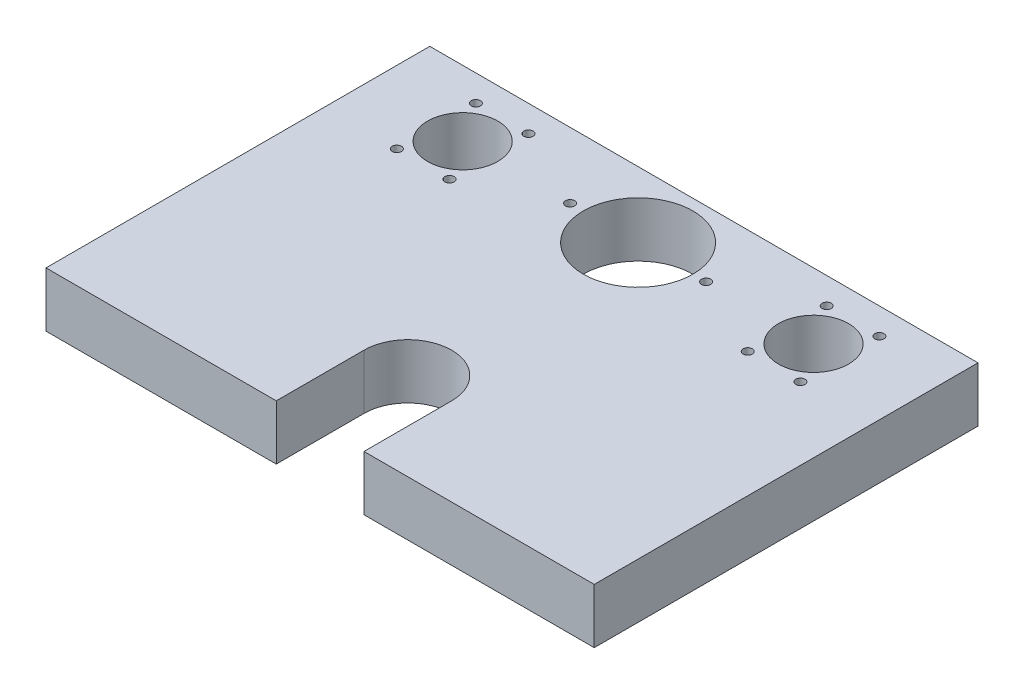
SolidWorks part; units mm, degrees
ref_plane "Front Plane" through (0, 0, 0) normal (0, 0, 1) x (1, 0, 0)
ref_plane "Top Plane" through (0, 0, 0) normal (0, 1, 0) x (1, 0, 0)
ref_plane "Right Plane" through (0, 0, 0) normal (1, 0, 0) x (0, 0, -1)
sketch "Sketch1" plane through (0, 0, 0) normal (0, 1, 0) x (1, 0, 0)
  line L1 (-125, 87.5) -> (125, 87.5)
  line L2 (-125, 87.5) -> (-125, -87.5)
  line L3 (-125, -87.5) -> (125, -87.5)
  line L4 (125, 87.5) -> (125, -87.5)
  line L5 (-125, 87.5) -> (125, -87.5) construction
  line L6 (-125, -87.5) -> (125, 87.5) construction
  point P0 (0, 0)
  dimension "D1" = 250
  dimension "D2" = 175
extrude "Boss-Extrude1" add sketch "Sketch1" along normal blind 25
sketch "Sketch2" plane through (0, 25, 0) normal (0, 1, 0) x (1, 0, 0)
  line L0 (-20, -47.5) -> (-20, -87.5)
  line L1 (-125, -87.5) -> (125, -87.5) construction
  line L2 (-20, -87.5) -> (20, -87.5)
  line L3 (20, -87.5) -> (20, -47.5)
  arc A0 (20, -47.5) -> (-20, -47.5) centre (0, -47.5) ccw
  dimension "D1" = 40
  dimension "D2" = 40
extrude "Cut-Extrude1" cut sketch "Sketch2" against normal through all
sketch "Sketch3" plane through (0, 25, 0) normal (0, 1, 0) x (1, 0, 0)
  line L0 (0, 0) -> (0, 48.5331) construction
  line L1 (125, 87.5) -> (-125, 87.5) construction
  circle A0 centre (-80, 57.5) radius 16
  circle A1 centre (80, 57.5) radius 16
  dimension "D1" = 32
  dimension "D2" = 30
  dimension "D3" = 80
extrude "Cut-Extrude2" cut sketch "Sketch3" against normal through all
sketch "Sketch4" plane through (0, 25, 0) normal (0, 1, 0) x (1, 0, 0)
  line L1 (-92, 39.5) -> (-68, 39.5) construction
  line L2 (-92, 39.5) -> (-92, 75.5) construction
  line L3 (-92, 75.5) -> (-68, 75.5) construction
  line L4 (-68, 39.5) -> (-68, 75.5) construction
  line L5 (-92, 39.5) -> (-68, 75.5) construction
  line L6 (-92, 75.5) -> (-68, 39.5) construction
  point P0 (-80, 57.5)
hole_wizard "M5 Tapped Hole2" positions "Sketch5" profile "Sketch6" tap size "M5" standard "GB"
sketch "Sketch5" plane through (0, 25, 0) normal (0, 1, 0) x (1, 0, 0)
  point P0 (-92, 75.5)
  point P3 (-68, 75.5)
  point P6 (-92, 39.5)
  point P9 (-68, 39.5)
sketch "Sketch6" plane through (-92, 25, -75.5) normal (1, 0, 0) x (0, 0, 1)
  line L0 (0, 0) -> (0, 13.6618)
  line L1 (0, 13.6618) -> (2.1, 12.4)
  line L2 (2.1, 12.4) -> (2.1, 0)
  line L5 (2.1, 0) -> (0, 0)
  line L10 (0, 13.6618) -> (-2.1, 12.4) construction
  line L11 (0, -6.35) -> (0, 107.95) construction
  dimension "螺纹孔钻头直径" = 4.2
  dimension "螺纹孔钻头深度" = 12.4
  dimension "导头角度" = 118
cosmetic thread "Cosmetic Thread1" parameters "D1"=10, "D2"=5
cosmetic thread "Cosmetic Thread2" parameters "D1"=10, "D2"=5
cosmetic thread "Cosmetic Thread3" parameters "D1"=10, "D2"=5
cosmetic thread "Cosmetic Thread4" parameters "D1"=10, "D2"=5
mirror "Mirror1" about plane through (0, 0, 0) normal (1, 0, 0) of "M5 Tapped Hole2"
sketch "Sketch7" plane through (0, 25, 0) normal (0, 1, 0) x (1, 0, 0)
  line L0 (-80, 57.5) -> (80, 57.5) construction
  circle A0 centre (0, 57.5) radius 25
  dimension "D1" = 50
extrude "Cut-Extrude3" cut sketch "Sketch7" against normal through all
sketch "Sketch8" plane through (0, 25, 0) normal (0, 1, 0) x (1, 0, 0)
  line L0 (-31, 57.5) -> (31, 57.5) construction
  point P4 (0, 57.5)
  dimension "D1" = 62
hole_wizard "M5 Tapped Hole1" positions "Sketch9" profile "Sketch10" tap size "M5" standard "GB" end condition through all
sketch "Sketch9" plane through (0, 25, 0) normal (0, 1, 0) x (1, 0, 0)
  point P0 (-31, 57.5)
  point P3 (31, 57.5)
sketch "Sketch10" plane through (-31, 25, -57.5) normal (1, 0, 0) x (0, 0, 1)
  line L0 (0, 0) -> (0, 25)
  line L1 (0, 25) -> (2.1, 25)
  line L2 (2.1, 25) -> (2.1, 0)
  line L5 (2.1, 0) -> (0, 0)
  line L11 (0, -6.35) -> (0, 107.95) construction
  dimension "通孔螺纹孔钻头直径" = 4.2
  dimension "通孔螺纹孔钻头深度" = 25
cosmetic thread "Cosmetic Thread5" parameters "D2"=5
cosmetic thread "Cosmetic Thread6" parameters "D2"=5
